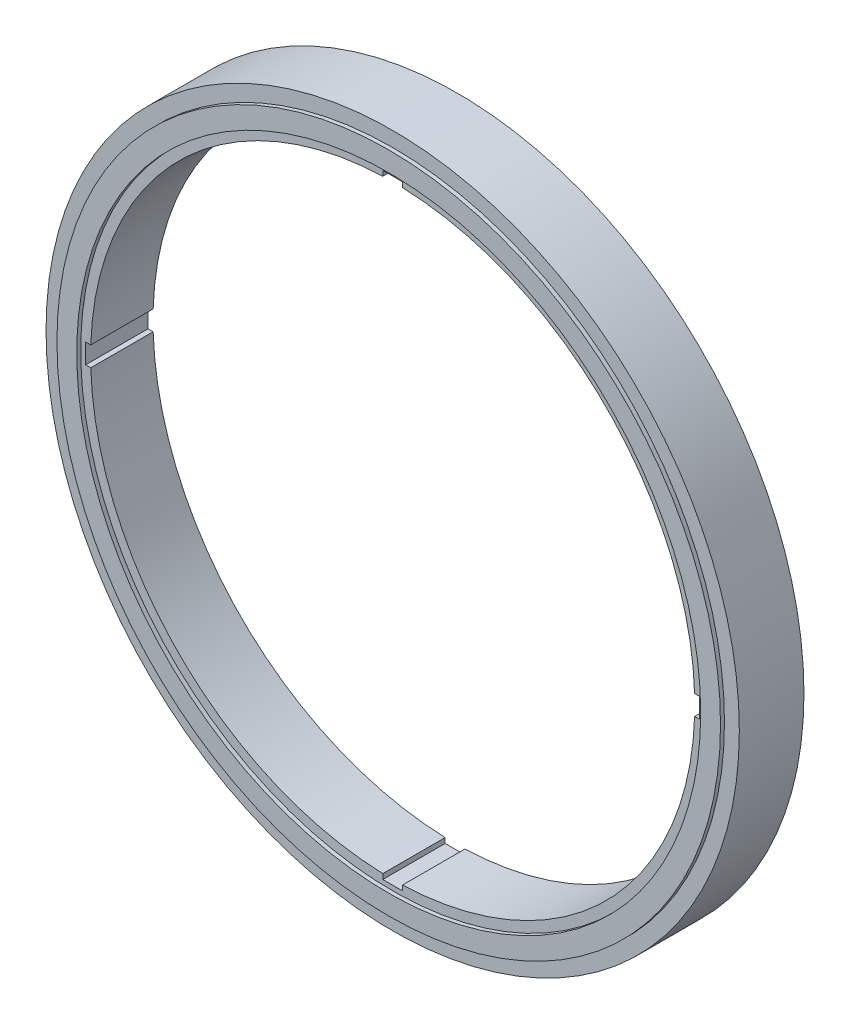
from build123d import *

# Parameters (mm, degrees)
SKETCH1_R           = 175
BOSS_EXTRUDE1_DEPTH = 35
CUT_EXTRUDE1_START  = -2
SKETCH2_R           = 175
SKETCH2_R_2         = 167.5
CUT_EXTRUDE1_DEPTH  = 2
SKETCH3_R           = 157.5
CUT_EXTRUDE2_DEPTH  = 2
SKETCH4_R           = 165
CUT_EXTRUDE3_DEPTH  = 1.5
SKETCH5_R           = 152.5
CUT_EXTRUDE4_DEPTH  = 250.744369306
SKETCH7_W           = 10
SKETCH7_H           = 310
CUT_EXTRUDE6_DEPTH  = 99.5
CIRPATTERN1_COUNT   = 4
SKETCH8_OUTSIDE_W   = 2071.968
SKETCH8_OUTSIDE_H   = 2071.968
SKETCH8_OUTSIDE_R   = 172
CUT_EXTRUDE7_DEPTH  = 99.5
CUT_EXTRUDE7_DRAFT  = -83


with BuildPart() as part:
    # Sketch1 → Boss-Extrude1 (new body)
    with BuildSketch(Plane.XY):
        Circle(SKETCH1_R)
    extrude(amount=BOSS_EXTRUDE1_DEPTH)

    # Sketch2 → Cut-Extrude1 (cut)
    with BuildSketch(Plane.XY.offset(35).offset(CUT_EXTRUDE1_START)):
        Circle(SKETCH2_R)
        Circle(SKETCH2_R_2, mode=Mode.SUBTRACT)
    extrude(amount=CUT_EXTRUDE1_DEPTH, mode=Mode.SUBTRACT)

    # Sketch3 → Cut-Extrude2 (cut)
    with BuildSketch(Plane.XY.offset(35)):
        Circle(SKETCH3_R)
    extrude(amount=-CUT_EXTRUDE2_DEPTH, mode=Mode.SUBTRACT)

    # Sketch4 → Cut-Extrude3 (cut)
    with BuildSketch(Plane(origin=(0, 0, 0), x_dir=(-1, 0, 0), z_dir=(0, 0, -1))):
        Circle(SKETCH4_R)
    extrude(amount=-CUT_EXTRUDE3_DEPTH, mode=Mode.SUBTRACT)

    # Sketch5 → Cut-Extrude4 (cut, through all)
    with BuildSketch(Plane(origin=(0, 0, 1.5), x_dir=(-1, 0, 0), z_dir=(0, 0, -1))):
        Circle(SKETCH5_R)
    extrude(amount=-CUT_EXTRUDE4_DEPTH, mode=Mode.SUBTRACT)

    # Sketch7 → Cut-Extrude6 (cut)
    with BuildSketch(Plane(origin=(0, 0, 1.5), x_dir=(-1, 0, 0), z_dir=(0, 0, -1))):
        Rectangle(SKETCH7_W, SKETCH7_H)
    cut_extrude6 = extrude(amount=-CUT_EXTRUDE6_DEPTH, mode=Mode.SUBTRACT)

    # CirPattern1: Cut-Extrude6 ×4 about axis
    cirpattern1_axis = Axis((0, 0, 0), (0, 0, 1))
    for i in range(1, CIRPATTERN1_COUNT):
        add(cut_extrude6.rotate(cirpattern1_axis, i * 360 / CIRPATTERN1_COUNT), mode=Mode.SUBTRACT)


with BuildPart() as cut_extrude7_tool:
    # Sketch8 outside → Cut-Extrude7 (with draft: the straight prism first)
    with BuildSketch(Plane(origin=(0, 0, 0), x_dir=(-1, 0, 0), z_dir=(0, 0, -1))):
        Rectangle(SKETCH8_OUTSIDE_W, SKETCH8_OUTSIDE_H)
        Circle(SKETCH8_OUTSIDE_R, mode=Mode.SUBTRACT)
    extrude(amount=-CUT_EXTRUDE7_DEPTH)
    # Cut-Extrude7: the draft: its side faces are tilted about the plane it starts from
    cut_extrude7_sides = [cut_extrude7_tool.faces().sort_by_distance(p)[0] for p in [
        (0, -1035.984, 49.75),
        (-1035.984, 0, 49.75),
        (0, 1035.984, 49.75),
        (1035.984, 0, 49.75),
        (172, 0, 49.75),
    ]]
    draft(cut_extrude7_sides, Plane(origin=(0, 0, 0), x_dir=(-1, 0, 0), z_dir=(0, 0, -1)), CUT_EXTRUDE7_DRAFT)


with BuildPart() as part_1:
    add(part.part)

    # Cut-Extrude7: cut by cut_extrude7_tool
    add(cut_extrude7_tool.part, mode=Mode.SUBTRACT)


solid = part_1.part
